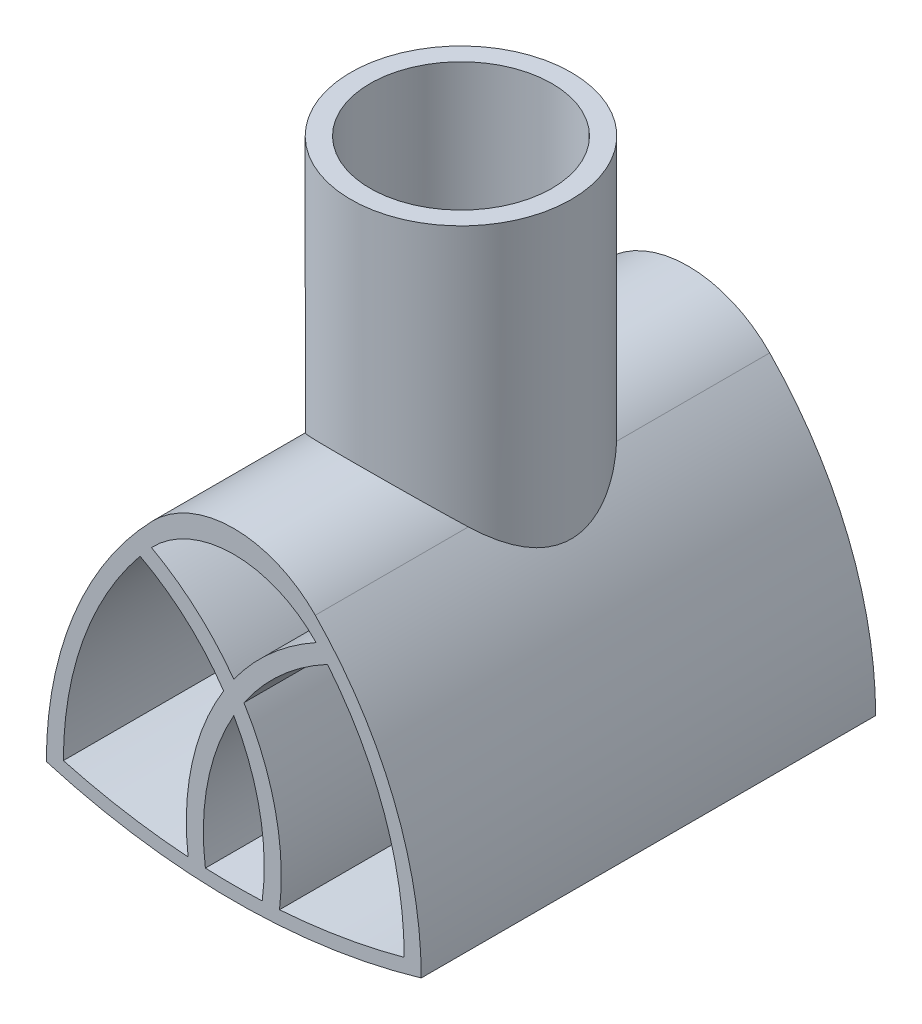
from build123d import *

# Parameters (mm, degrees)
EXTRUDE_1182_DEPTH                  = 20
SKETCH_1261_R                       = 9.7
SKETCH_1261_R_2                     = 8
EXTRUDE_1314_DEPTH                  = 25
EXTRUDE_1314_DIRECTION_2_REACH      = 36.873
EXTRUDE_1314_DIRECTION_2_END_RADIUS = 57.25
CUT_EXTRUDE_1_DEPTH                 = 54.783006673
CUT_EXTRUDE_1_DEPTH_BACK            = 54.783006673


with BuildPart() as part:
    # Sketch 176 → Extrude 1182 (new, symmetric)
    with BuildSketch(Plane.XY):
        with BuildLine():
            ThreePointArc((-7.173913043, 24.16738193), (-14.079724741, 13.582112358), (-16.5, 1.177257067))
            ThreePointArc((-16.5, 1.177257067), (0, -1.2), (16.5, 1.177257067))
            ThreePointArc((16.5, 1.177257067), (14.079724741, 13.582112358), (7.173913043, 24.16738193))
            ThreePointArc((7.173913043, 24.16738193), (0, 27.200677426), (-7.173913043, 24.16738193))
        make_face()
        with BuildLine():
            ThreePointArc((-0.89349881, 14.363604773), (-3.663033007, 7.517669831), (-4.022846329, 0.141513701))
            ThreePointArc((-4.022846329, 0.141513701), (-9.556707772, 0.803283208), (-15, 2))
            ThreePointArc((-15, 2), (-13.262165522, 12.062305899), (-8.25, 20.95883699))
            ThreePointArc((-8.25, 20.95883699), (-4.170568058, 18.108709455), (-0.89349881, 14.363604773))
        make_face(mode=Mode.SUBTRACT)
        with BuildLine():
            ThreePointArc((-2.5, 0.0546112), (-2.301572456, 6.695550977), (0, 12.928064021))
            ThreePointArc((0, 12.928064021), (2.301572456, 6.695550977), (2.5, 0.0546112))
            ThreePointArc((2.5, 0.0546112), (0, 0), (-2.5, 0.0546112))
        make_face(mode=Mode.SUBTRACT)
        with BuildLine():
            ThreePointArc((4.022846329, 0.141513701), (3.663033007, 7.517669831), (0.89349881, 14.363604773))
            ThreePointArc((0.89349881, 14.363604773), (4.170568058, 18.108709455), (8.25, 20.95883699))
            ThreePointArc((8.25, 20.95883699), (13.262165522, 12.062305899), (15, 2))
            ThreePointArc((15, 2), (9.556707772, 0.803283208), (4.022846329, 0.141513701))
        make_face(mode=Mode.SUBTRACT)
        with BuildLine():
            ThreePointArc((7.245751005, 22.120715085), (3.267177029, 19.312833939), (0, 15.701905849))
            ThreePointArc((0, 15.701905849), (-3.267177029, 19.312833939), (-7.245751005, 22.120715085))
            ThreePointArc((-7.245751005, 22.120715085), (0, 25.228756555), (7.245751005, 22.120715085))
        make_face(mode=Mode.SUBTRACT)
    extrude(amount=EXTRUDE_1182_DEPTH, both=True)

    # Sketch 1261 → Extrude 1314 (add)
    with BuildSketch(Plane(origin=(0, 22.120715085, 0), x_dir=(-1, 0, 0), z_dir=(0, -1, 0))):
        with Locations(Location((0, 0, 0), (0, 0, 222.304463408))):
            Circle(SKETCH_1261_R)
        with Locations(Location((0, 0, 0), (0, 0, 206.267303198))):
            Circle(SKETCH_1261_R_2, mode=Mode.SUBTRACT)
    extrude(amount=-EXTRUDE_1314_DEPTH)

    # Extrude 1314 direction 2: up to this cylinder (the profile starts inside it)
    extrude_1314_direction_2_end = Plane(origin=(0, 57.25, -6.344118), z_dir=(0, 0, -1)) * Cylinder(EXTRUDE_1314_DIRECTION_2_END_RADIUS, 189.246, mode=Mode.PRIVATE)
    # Sketch 1261 → Extrude 1314 direction 2 (add, up to the surface)
    with BuildSketch(Plane(origin=(0, 22.120715085, 0), x_dir=(-1, 0, 0), z_dir=(0, -1, 0)), mode=Mode.PRIVATE) as extrude_1314_direction_2_sk1:
        with Locations(Location((0, 0, 0), (0, 0, 222.304463408))):
            Circle(SKETCH_1261_R)
        with Locations(Location((0, 0, 0), (0, 0, 206.267303198))):
            Circle(SKETCH_1261_R_2, mode=Mode.SUBTRACT)
    extrude_1314_direction_2_tool1 = extrude(extrude_1314_direction_2_sk1.sketch, amount=EXTRUDE_1314_DIRECTION_2_REACH, mode=Mode.PRIVATE) & extrude_1314_direction_2_end
    add(extrude_1314_direction_2_tool1.solids().sort_by_distance((-6.971004, 22.120715, -6.344118))[0])

    # Sketch 1375 → 切除-拉伸1 (cut, two sides: drawn at the far end of the back side and taken through both)
    with BuildSketch(Plane.XY.offset(-CUT_EXTRUDE_1_DEPTH_BACK)):
        with BuildLine():
            ThreePointArc((4.022846329, 0.141513701), (9.556707772, 0.803283208), (15, 2))
            ThreePointArc((15, 2), (13.262165522, 12.062305899), (8.25, 20.95883699))
            ThreePointArc((8.25, 20.95883699), (4.170568058, 18.108709455), (0.89349881, 14.363604773))
            ThreePointArc((0.89349881, 14.363604773), (3.663033007, 7.517669831), (4.022846329, 0.141513701))
        make_face()
        with BuildLine():
            ThreePointArc((-8.25, 20.95883699), (-13.262165522, 12.062305899), (-15, 2))
            ThreePointArc((-15, 2), (-9.556707772, 0.803283208), (-4.022846329, 0.141513701))
            ThreePointArc((-4.022846329, 0.141513701), (-3.663033007, 7.517669831), (-0.89349881, 14.363604773))
            ThreePointArc((-0.89349881, 14.363604773), (-4.170568058, 18.108709455), (-8.25, 20.95883699))
        make_face()
        with BuildLine():
            ThreePointArc((-2.5, 0.0546112), (0, 0), (2.5, 0.0546112))
            ThreePointArc((2.5, 0.0546112), (2.301572456, 6.695550977), (0, 12.928064021))
            ThreePointArc((0, 12.928064021), (-2.301572456, 6.695550977), (-2.5, 0.0546112))
        make_face()
        with BuildLine():
            ThreePointArc((7.245751005, 22.120715085), (3.267177029, 19.312833939), (0, 15.701905849))
            ThreePointArc((0, 15.701905849), (-3.267177029, 19.312833939), (-7.245751005, 22.120715085))
            ThreePointArc((-7.245751005, 22.120715085), (0, 25.228756555), (7.245751005, 22.120715085))
        make_face()
    extrude(amount=CUT_EXTRUDE_1_DEPTH + CUT_EXTRUDE_1_DEPTH_BACK, mode=Mode.SUBTRACT)


solid = part.part
